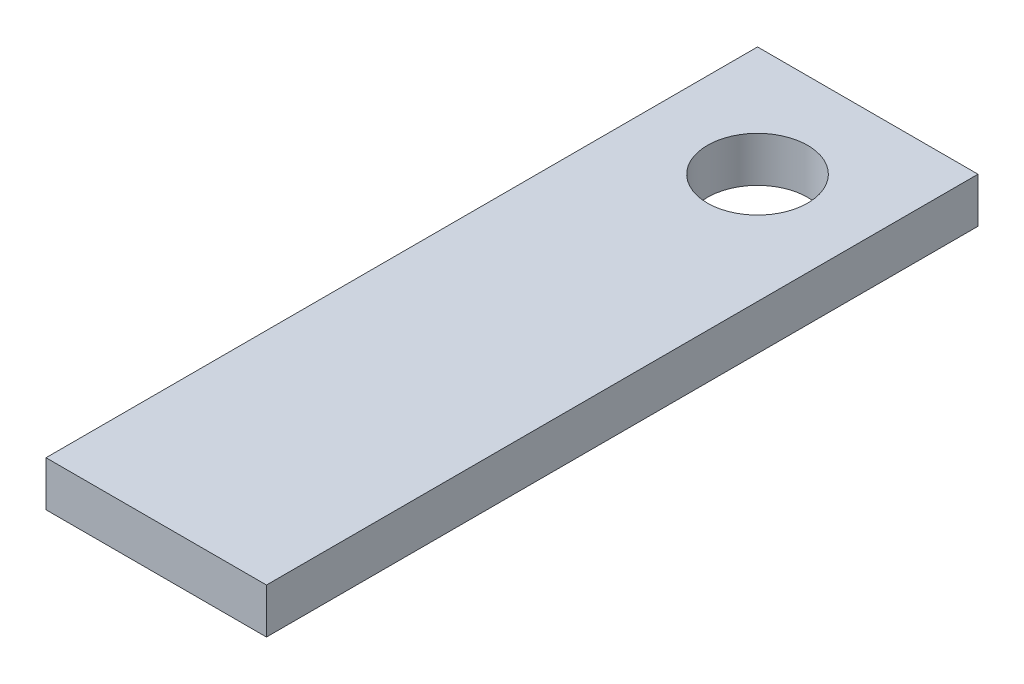
SolidWorks part; units mm, degrees
ref_plane "Front Plane" through (0, 0, 0) normal (0, 0, 1) x (1, 0, 0)
ref_plane "Top Plane" through (0, 0, 0) normal (0, 1, 0) x (1, 0, 0)
ref_plane "Right Plane" through (0, 0, 0) normal (1, 0, 0) x (0, 0, -1)
sketch "Sketch1" plane through (0, 0, 0) normal (0, 1, 0) x (1, 0, 0)
  line L1 (0, 0) -> (22, 0)
  line L2 (0, 0) -> (0, 71)
  line L3 (0, 71) -> (22, 71)
  line L4 (22, 0) -> (22, 71)
  circle A0 centre (11, 60) radius 5
  dimension "D3" = 11
  dimension "D4" = 11
  dimension "D5" = 10
  dimension "D1" = 22
  dimension "D2" = 71
extrude "Boss-Extrude1" add sketch "Sketch1" along normal blind 4.5
